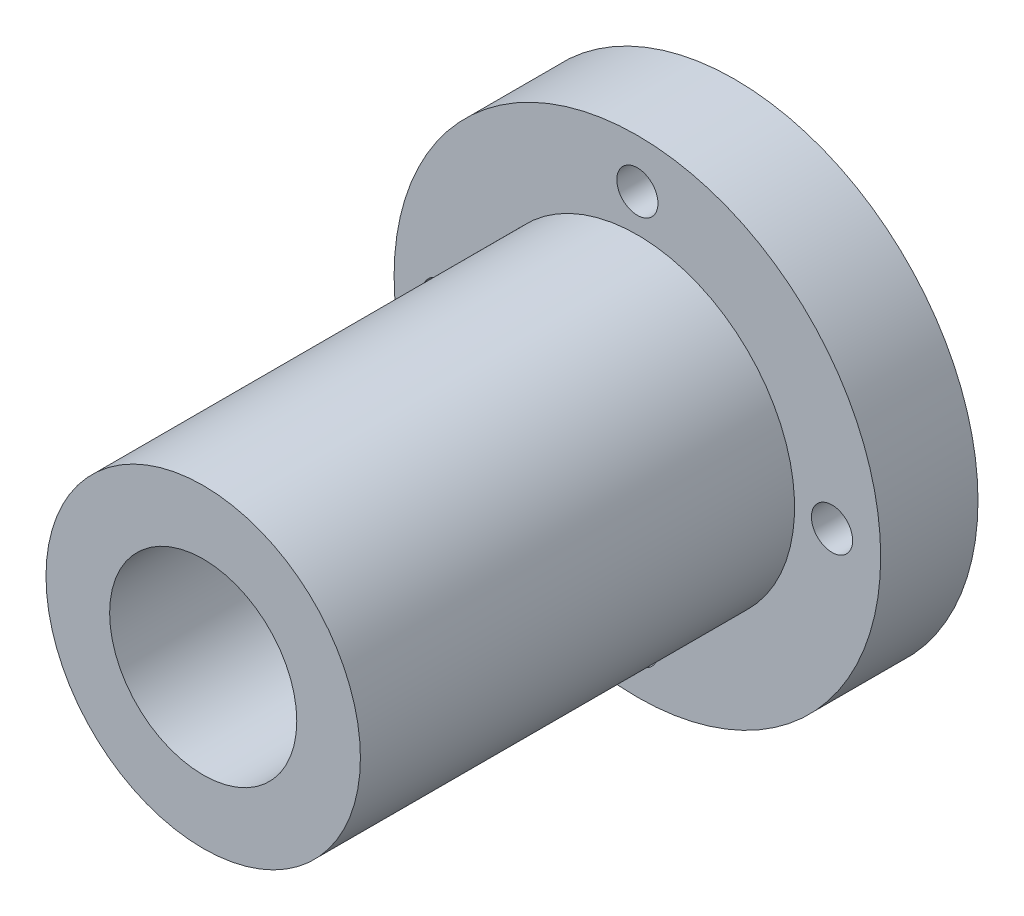
SolidWorks part; units mm, degrees
ref_plane "前视基准面" through (0, 0, 0) normal (0, 0, 1) x (1, 0, 0)
ref_plane "上视基准面" through (0, 0, 0) normal (0, 1, 0) x (1, 0, 0)
ref_plane "右视基准面" through (0, 0, 0) normal (1, 0, 0) x (0, 0, -1)
sketch "草图1" plane through (0, 0, 0) normal (0, 0, 1) x (1, 0, 0)
  circle A0 centre (0, 0) radius 12.5
  circle A1 centre (0, 0) radius 21
  dimension "D1" = 25
  dimension "D2" = 42
extrude "凸台-拉伸1" add sketch "草图1" along normal blind 71
sketch "草图2" plane through (0, 0, 0) normal (0, 0, -1) x (-1, 0, 0)
  circle A0 centre (0, 0) radius 12.5 construction
  circle A1 centre (0, 0) radius 12.5
  circle A2 centre (0, 0) radius 32.5
  dimension "D1" = 65
extrude "凸台-拉伸2" add sketch "草图2" against normal blind 13
sketch "草图5" plane through (0, 0, 0) normal (0, 0, 1) x (1, 0, 0)
  circle A0 centre (0, 0) radius 26
  point P3 (0, 26)
  point P4 (26, 0)
  point P5 (0, -26)
  point P6 (-26, 0)
  dimension "D1" = 52
hole_wizard "打孔尺寸(%根据)内六角圆柱头螺钉的类型1" positions "3D草图3" profile "草图7" counterbore size "M5" standard "GB" end condition up to next
sketch3d "3D草图3"
  point P0 (0, 26, 0)
  point P3 (-26, 0, 0)
  point P6 (0, -26, 0)
  point P9 (26, 0, 0)
sketch "草图7" plane through (0, 26, 0) normal (1, 0, 0) x (0, 1, 0)
  line L0 (0, 0) -> (0, 13)
  line L1 (0, 13) -> (2.75, 13)
  line L3 (2.75, 13) -> (2.75, 5.7)
  line L4 (2.75, 5.7) -> (5, 5.7)
  line L5 (5, 5.7) -> (5, 0)
  line L7 (5, 0) -> (0, 0)
  line L11 (0, -6.35) -> (0, 107.95) construction
  dimension "通孔孔直径" = 5.5
  dimension "通孔孔深度" = 13
  dimension "柱形沉头孔直径" = 10
  dimension "柱形沉头孔深度" = 5.7
sketch "草图8" plane through (0, 0, 0) normal (0, 0, -1) x (-1, 0, 0)
  circle A0 centre (0, 0) radius 27.5
  dimension "D1" = 55
